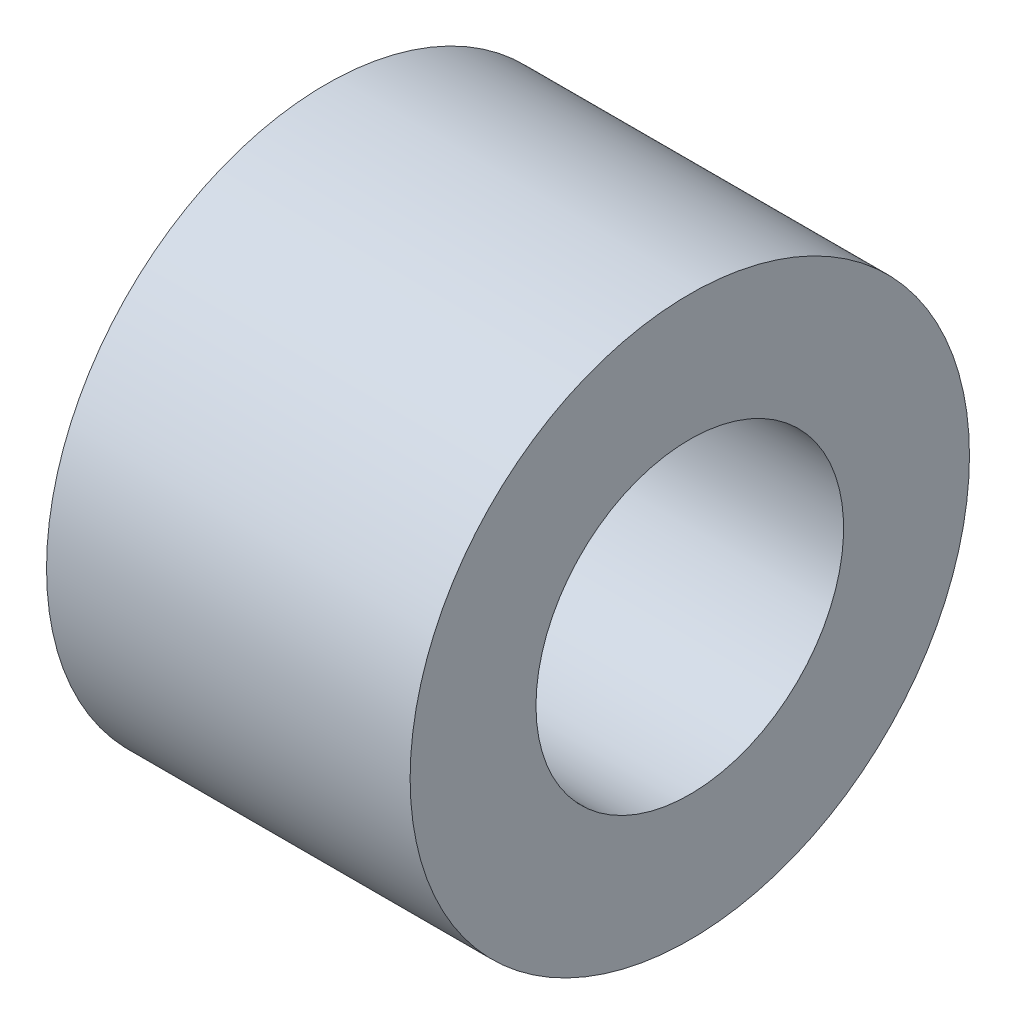
SolidWorks part; units mm, degrees
material "Q235A"
ref_plane "Front Plane" through (0, 0, 0) normal (0, 0, 1) x (1, 0, 0)
ref_plane "Top Plane" through (0, 0, 0) normal (0, 1, 0) x (1, 0, 0)
ref_plane "Right Plane" through (0, 0, 0) normal (1, 0, 0) x (0, 0, -1)
sketch "Sketch2" plane through (0, 0, 0) normal (1, 0, 0) x (0, 0, -1)
  circle A0 centre (0, 0) radius 5.5
  circle A1 centre (0, 0) radius 10
  dimension "D1" = 11
  dimension "D2" = 20
extrude "Boss-Extrude2" add sketch "Sketch2" along normal mid plane 13
